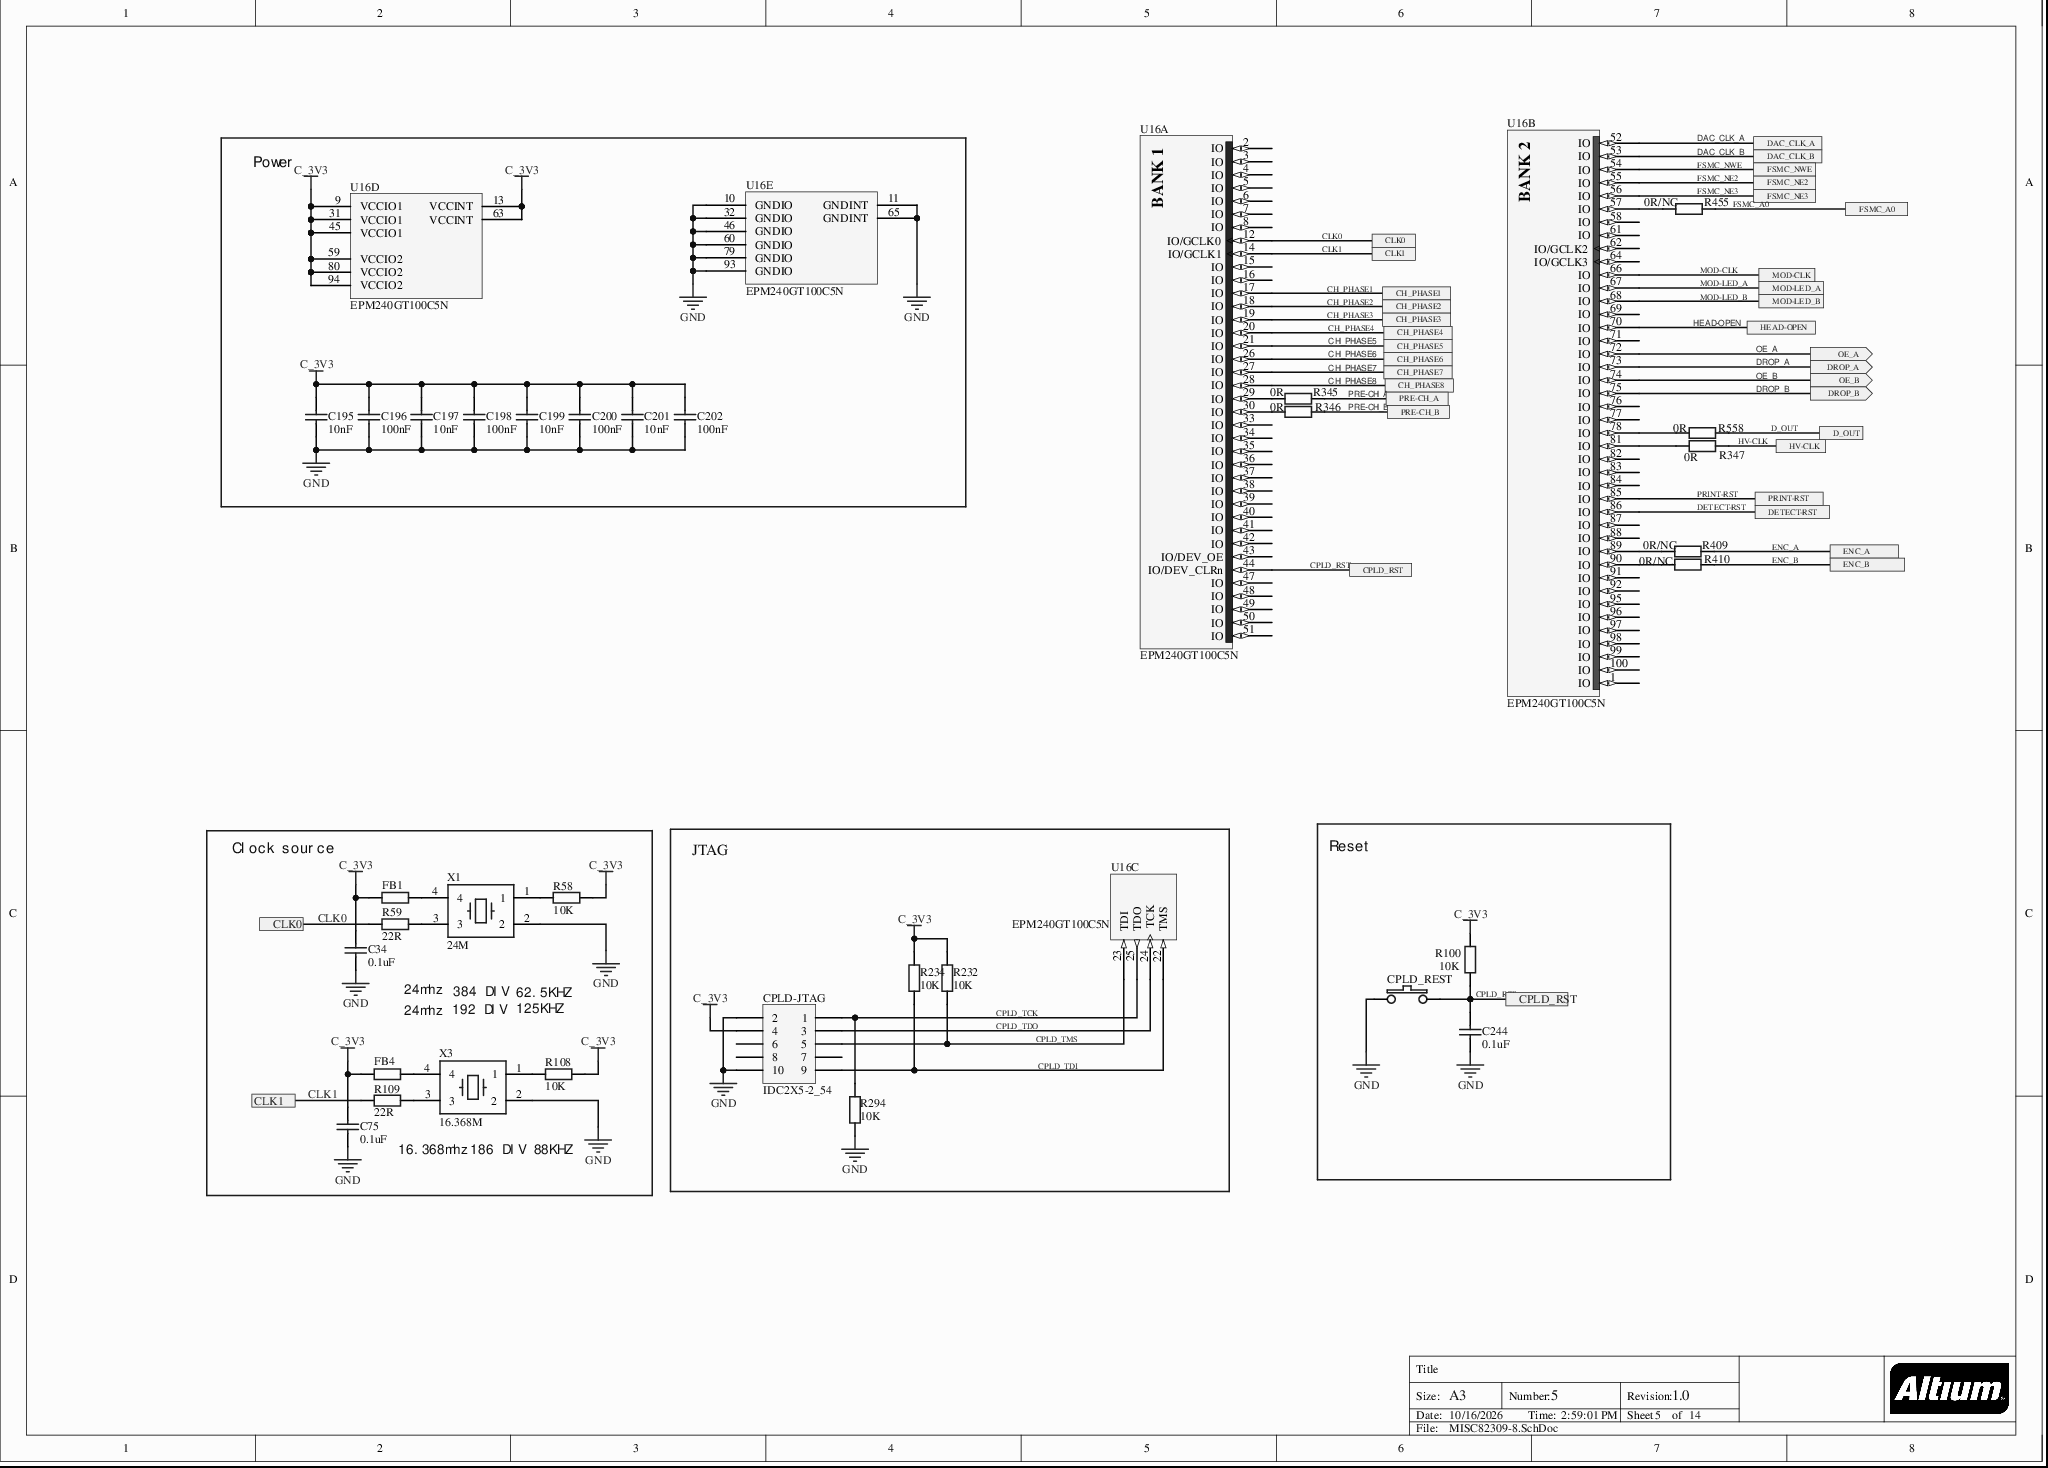
[diagram p0: MISC82309-8.SchDoc]
# Altium project MISC82309-16.PrjPcb (part 3 of 6)

## Sheet MISC82309-8.SchDoc
size A3; DocumentNumber: 5; Revision: 1.0; SheetNumber: 5; SheetTotal: 14

### Parts
C34  0.1uF  [C0603]
C75  0.1uF  [C0603]
C195  10nF  [C0805]
C196  100nF  [C0805]
C197  10nF  [C0805]
C198  100nF  [C0805]
C199  10nF  [C0805]
C200  100nF  [C0805]
C201  10nF  [C0805]
C202  100nF  [C0805]
C244  0.1uF  [C0603]
CPLD-JTAG  IDC2X5-2_54  [IDC2X5-2_54]
CPLD_REST  SW  [SW-6X3X2.5]  (value not drawn)
FB1  60  [SMD1206-L]  (value not drawn)
FB4  60  [SMD1206-L]  (value not drawn)
R58  10K  [R0603]
R59  22R  [R0603]
R100  10K  [R0603]
R108  10K  [R0603]
R109  22R  [R0603]
R232  10K  [R0603]
R234  10K  [R0603]
R294  10K  [R0603]
R345  0R  [RES_0603]
R346  0R  [RES_0603]
R347  0R  [RES_0603]
R409  0R/NC  [RES_0603]
R410  0R/NC  [RES_0603]
R455  0R/NC  [RES_0603]
R558  0R  [RES_0603]
U16  EPM240GT100C5N  [TQFP100_N]  (parts A,B,C,D,E of 5)
X1  24M  [SMD5032]
X3  16.368M  [SMD5032]

### Blocks framed on the sheet
Power: C195-C202 U16
Clock source: C34 C75 FB1 FB4 R58 R59 R108 R109 X1 X3
JTAG: CPLD-JTAG R232 R234 R294 U16
Reset: C244 CPLD_REST R100

### Ports
CH_PHASE1, CH_PHASE2, CH_PHASE3, CH_PHASE4, CH_PHASE5, CH_PHASE6, CH_PHASE7, CH_PHASE8, CLK0, CLK1, CPLD_RST, D_OUT, DAC_CLK_A, DAC_CLK_B, DETECT-RST, DROP_A (out), DROP_B (out), ENC_A, ENC_B, FSMC_A0, FSMC_NE2, FSMC_NE3, FSMC_NWE, HEAD-OPEN, HV-CLK, MOD-CLK, MOD-LED_A, MOD-LED_B, OE_A (out), OE_B (out), PRE-CH_A, PRE-CH_B, PRINT-RST

### Nets
C_3V3: C34.2 C75.2 C195.2 C196.2 C197.2 C198.2 C199.2 C200.2 C201.2 C202.2 CPLD-JTAG.4 FB1.1 FB4.1 R58.2 R100.1 R108.2 R232.2 R234.2 U16.9(VCCIO1) U16.13(VCCINT) U16.31(VCCIO1) U16.45(VCCIO1) U16.59(VCCIO2) U16.63(VCCINT) U16.80(VCCIO2) U16.94(VCCIO2)
GND: C34.1 C75.1 C195.1 C196.1 C197.1 C198.1 C199.1 C200.1 C201.1 C202.1 C244.1 CPLD-JTAG.2 CPLD-JTAG.10 CPLD_REST.1 R294.1 U16.10(GNDIO) U16.11(GNDINT) U16.32(GNDIO) U16.46(GNDIO) U16.60(GNDIO) U16.65(GNDINT) U16.79(GNDIO) U16.93(GNDIO) X1.2 X3.2
CH_PHASE1: U16.17(IO) ; port CH_PHASE1
CH_PHASE2: U16.18(IO) ; port CH_PHASE2
CH_PHASE3: U16.19(IO) ; port CH_PHASE3
CH_PHASE4: U16.20(IO) ; port CH_PHASE4
CH_PHASE5: U16.21(IO) ; port CH_PHASE5
CH_PHASE6: U16.26(IO) ; port CH_PHASE6
CH_PHASE7: U16.27(IO) ; port CH_PHASE7
CH_PHASE8: U16.28(IO) ; port CH_PHASE8
CLK0: R59.1 U16.12(IO/GCLK0) ; port CLK0
CLK1: R109.1 U16.14(IO/GCLK1) ; port CLK1
CPLD_RST: C244.2 CPLD_REST.2 R100.2 U16.44(IO/DEV_CLRn) ; port CPLD_RST
CPLD_TCK: CPLD-JTAG.1 R294.2 U16.25(TDO)
CPLD_TDI: CPLD-JTAG.9 R234.1 U16.22(TMS)
CPLD_TDO: CPLD-JTAG.3 U16.24(TCK)
CPLD_TMS: CPLD-JTAG.5 R232.1 U16.23(TDI)
D_OUT: R558.1 ; port D_OUT
DAC_CLK_A: U16.52(IO) ; port DAC_CLK_A
DAC_CLK_B: U16.53(IO) ; port DAC_CLK_B
DETECT-RST: U16.86(IO) ; port DETECT-RST
DROP_A: U16.73(IO) ; port DROP_A
DROP_B: U16.75(IO) ; port DROP_B
ENC_A: R409.2 ; port ENC_A
ENC_B: R410.2 ; port ENC_B
FSMC_A0: R455.2 ; port FSMC_A0
FSMC_NE2: U16.55(IO) ; port FSMC_NE2
FSMC_NE3: U16.56(IO) ; port FSMC_NE3
FSMC_NWE: U16.54(IO) ; port FSMC_NWE
HEAD-OPEN: U16.70(IO) ; port HEAD-OPEN
HV-CLK: R347.2 ; port HV-CLK
MOD-CLK: U16.66(IO) ; port MOD-CLK
MOD-LED_A: U16.67(IO) ; port MOD-LED_A
MOD-LED_B: U16.68(IO) ; port MOD-LED_B
OE_A: U16.72(IO) ; port OE_A
OE_B: U16.74(IO) ; port OE_B
PRE-CH_A: R345.2 ; port PRE-CH_A
PRE-CH_B: R346.2 ; port PRE-CH_B
PRINT-RST: U16.85(IO) ; port PRINT-RST
NetFB1_2: FB1.2 X1.4
NetFB4_2: FB4.2 X3.4
NetR58_1: R58.1 X1.1
NetR59_2: R59.2 X1.3
NetR108_1: R108.1 X3.1
NetR109_2: R109.2 X3.3
NetR345_1: R345.1 U16.29(IO)
NetR346_1: R346.1 U16.30(IO)
NetR347_1: R347.1 U16.81(IO)
NetR409_1: R409.1 U16.89(IO)
NetR410_1: R410.1 U16.90(IO)
NetR455_1: R455.1 U16.57(IO)
NetR558_2: R558.2 U16.78(IO)

Not connected (* = marked no-connect by the designer): CPLD-JTAG 6 7 8; CPLD_REST 5 6; U16 1(IO) 2(IO) 3(IO) 4(IO) 5(IO) 6(IO) 7(IO) 8(IO) 15(IO) 16(IO) 33(IO) 34(IO) 35(IO) 36(IO) 37(IO) 38(IO) 39(IO) 40(IO) 41(IO) 42(IO) 43(IO/DEV_OE) 47(IO) 48(IO) 49(IO) 50(IO) 51(IO) 58(IO) 61(IO) 62(IO/GCLK2) 64(IO/GCLK3) 69(IO) 71(IO) 76(IO) 77(IO) 82(IO) 83(IO) 84(IO) 87(IO) 88(IO) 91(IO) 92(IO) 95(IO) 96(IO) 97(IO) 98(IO) 99(IO) 100(IO)

### Notes on the sheet
- 24mhz
- 192 DIV
- 384 DIV
- 125KHZ
- 62.5KHZ
- 16.368mhz
- (near X3) 186 DIV
- 88KHZ
- Title
- Size:
- Date:
- A3
- Number:
- Time:
- Revision:
- Sheet
- of
- File:

### Library data of the parts
C34 C75 C195 C197 C199 C201 C244 = CAP_1206: Capacitor
  C34 C75 C244: value: 0.1uF
  C195 C197 C199 C201: value: 10nF
C196 C198 C200 C202 = CAP_1206: Capacitor; value: 0.1uF
CPLD-JTAG = HEAD2X5-2_54
FB1 FB4 = FB: Res; value: 10K
R58 R108 R232 R234 R294 = Res: value: 10K
R59 R109 = Res: value: 22ohm
R100 = Res2: Resistor; Published: 8-Jun-2000; LatestRevisionDate: 17-Jul-2002; LatestRevisionNote: Re-released for DXP Platform.; PackageReference: AXIAL-0.4; Value: 10K; Publisher: Altium Limited
R345-R347 = Res_0603: Res; value: 0R
R409 R410 R455 = Res_0603: Res; value: 0R
R558 = Res_0603: Res; value: 0R/NC
U16 = EPM240GT100C5N: MAX II 1.8V CPLD, 80 IOs, 240 Logic Elements, 100-Pin Plastic TQFP, Commercial Temperature, Speed Grade 5, Pb-Free; Note: Each set of VCCIO pins can be connected to 3.3V, 2.5V, 1.8V, or 1.5V.; Note: All VCCINT pins must be connected to 1.8V.; Published: 4-Mar-2005; LatestRevisionDate: 13-Apr-2006; LatestRevisionNote: IPC-7351 Footprint Added.; DatasheetVersion: ver1.8, Jul-2006; PackageVersion: ver14.3, Jul-2006; PackageReference: TQFP100; PackageDescription: 100-Pin Plastic Thin Quad Flat Pack (TQFP100); Code_JEDEC: MS-026-AED; ComponentLink1Description: Manufacturer Link; ComponentLink1URL: http://www.altera.com/products/devices/cpld/max2/mx2-index.jsp; ComponentLink2Description: Handbook; ComponentLink2URL: http://www.altera.com/literature/hb/max2/max2_mii5v1.pdf; ComponentLink3Description: Packaging Specification; ComponentLink3URL: http://www.altera.com/literature/ds/dspkg.pdf; Publisher: Altium Limited
X1 X3 = SOC_24M

## Sheet MISC82309-13.SchDoc
size A3; DocumentNumber: 6; Revision: 1.0; SheetNumber: 6; SheetTotal: 14
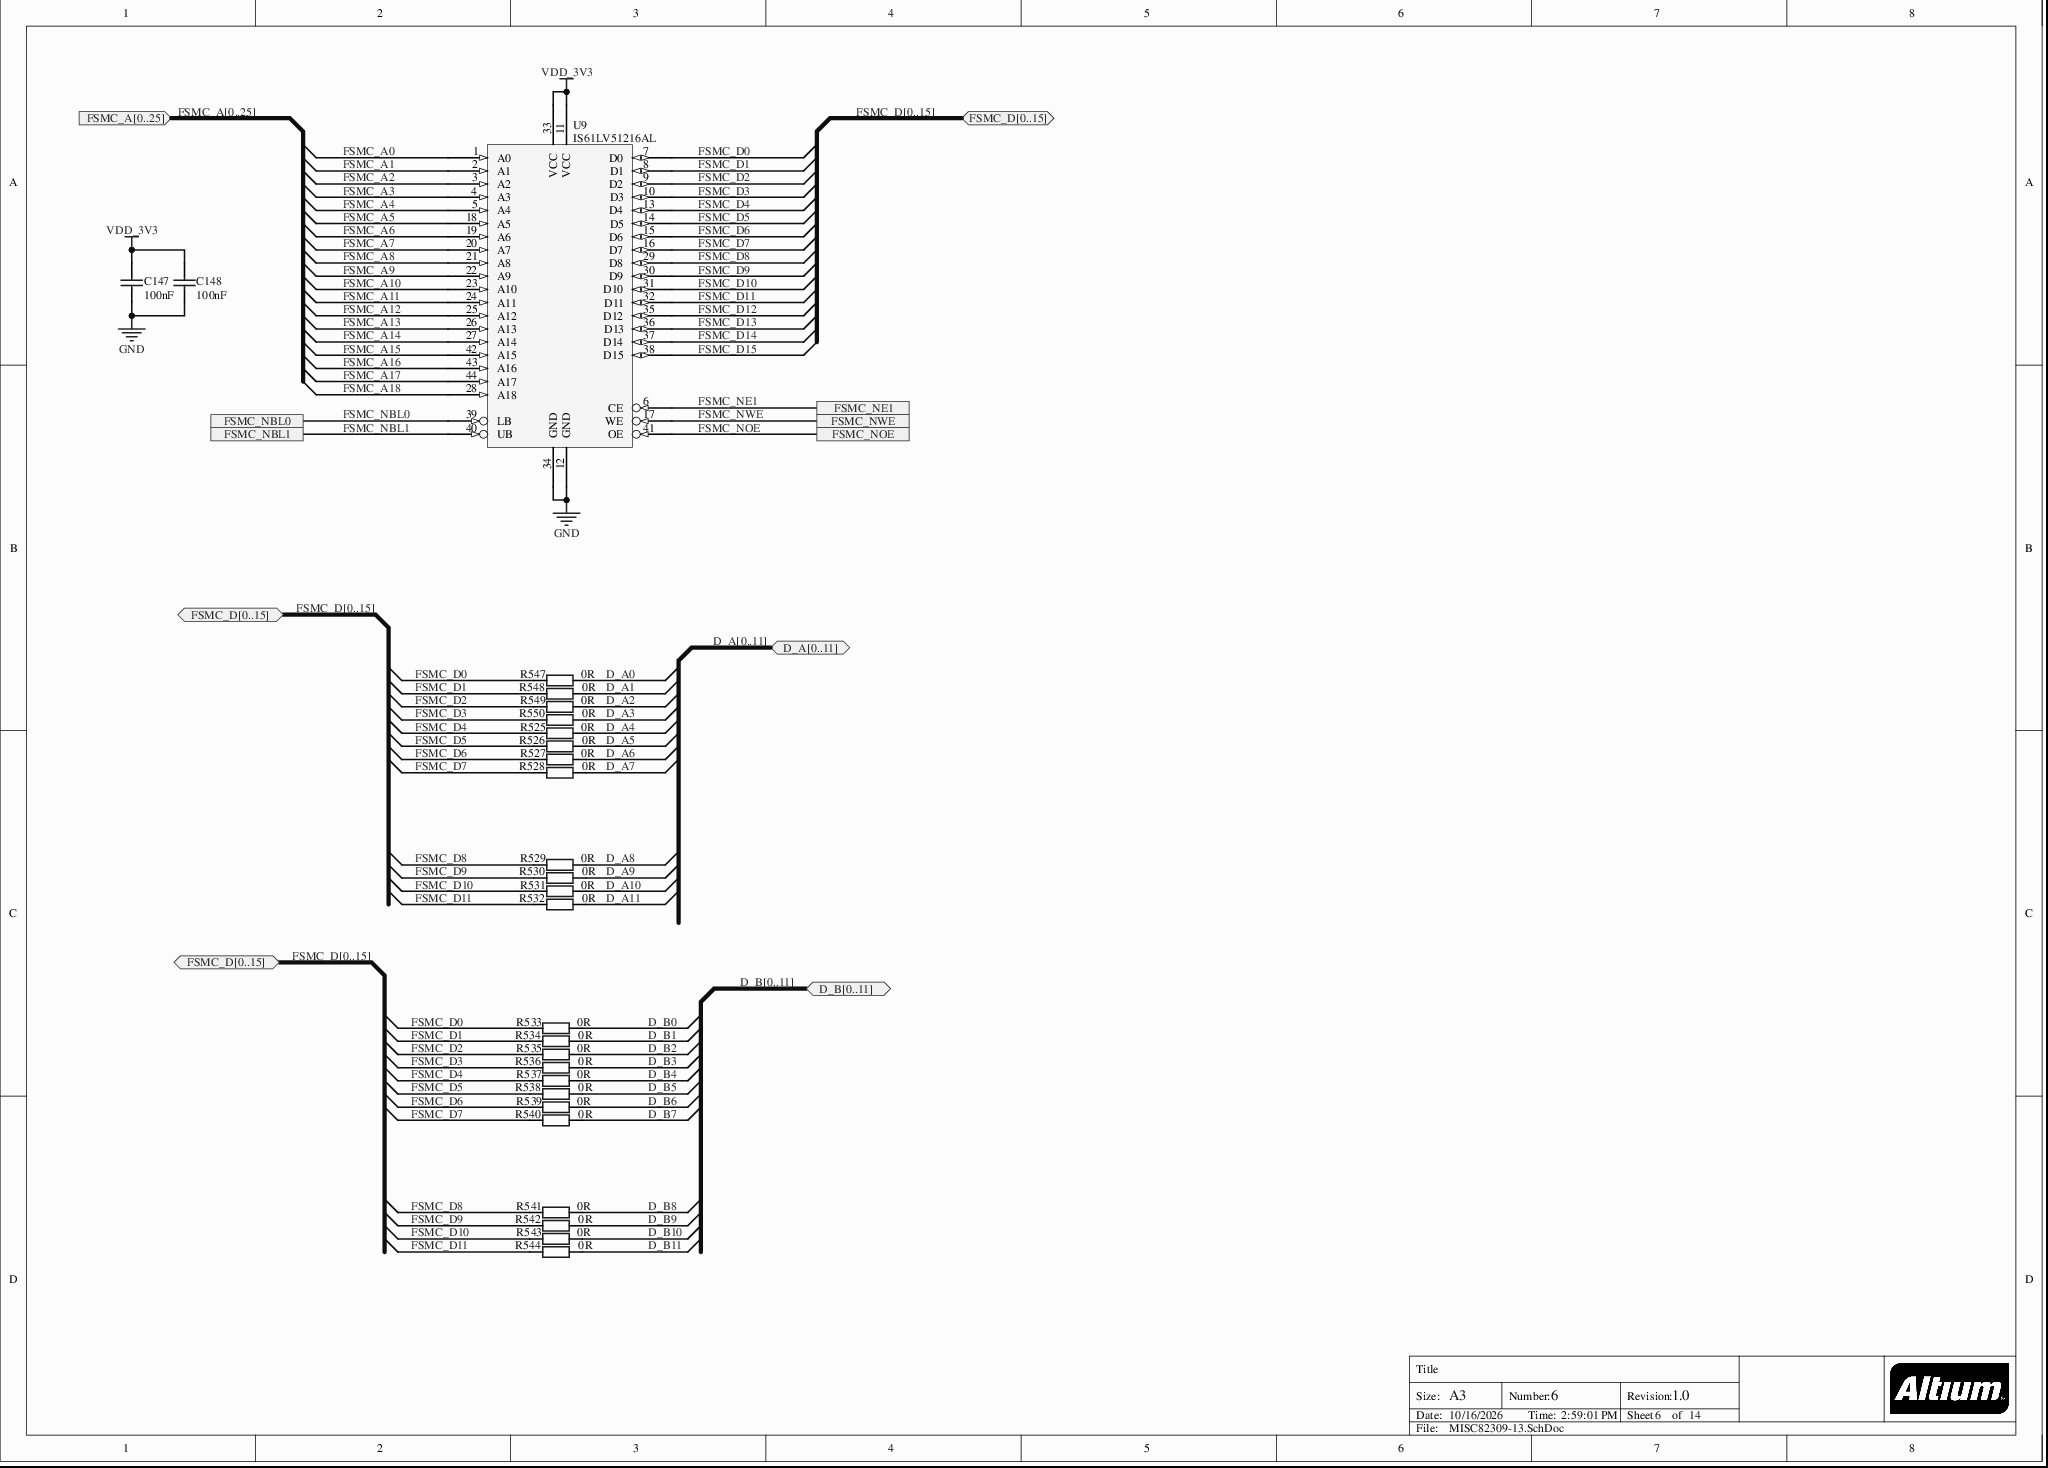
[diagram p1: MISC82309-13.SchDoc]

### Parts
C147  100nF  [C0603]
C148  100nF  [C0603]
R525  0R  [RES_0603]
R526  0R  [RES_0603]
R527  0R  [RES_0603]
R528  0R  [RES_0603]
R529  0R  [RES_0603]
R530  0R  [RES_0603]
R531  0R  [RES_0603]
R532  0R  [RES_0603]
R533  0R  [RES_0603]
R534  0R  [RES_0603]
R535  0R  [RES_0603]
R536  0R  [RES_0603]
R537  0R  [RES_0603]
R538  0R  [RES_0603]
R539  0R  [RES_0603]
R540  0R  [RES_0603]
R541  0R  [RES_0603]
R542  0R  [RES_0603]
R543  0R  [RES_0603]
R544  0R  [RES_0603]
R547  0R  [RES_0603]
R548  0R  [RES_0603]
R549  0R  [RES_0603]
R550  0R  [RES_0603]
U9  IS61LV51216AL  [TSOP44-IS61LV51216AL-10TLI]

### Ports
D_A[0..11] (bidir), D_B[0..11] (bidir), FSMC_A[0..25] (in), FSMC_D[0..15] (bidir), FSMC_NBL0, FSMC_NBL1, FSMC_NE1, FSMC_NOE, FSMC_NWE

### Nets
GND: C147.1 C148.1 U9.12(GND) U9.34(GND)
VDD_3V3: C147.2 C148.2 U9.11(VCC) U9.33(VCC)
D_A0: R547.1
D_A1: R548.1
D_A2: R549.1
D_A3: R550.1
D_A4: R525.1
D_A5: R526.1
D_A6: R527.1
D_A7: R528.1
D_A8: R529.1
D_A9: R530.1
D_A10: R531.1
D_A11: R532.1
D_B0: R533.1
D_B1: R534.1
D_B2: R535.1
D_B3: R536.1
D_B4: R537.1
D_B5: R538.1
D_B6: R539.1
D_B7: R540.1
D_B8: R541.1
D_B9: R542.1
D_B10: R543.1
D_B11: R544.1
FSMC_A0: U9.1(A0)
FSMC_A1: U9.2(A1)
FSMC_A2: U9.3(A2)
FSMC_A3: U9.4(A3)
FSMC_A4: U9.5(A4)
FSMC_A5: U9.18(A5)
FSMC_A6: U9.19(A6)
FSMC_A7: U9.20(A7)
FSMC_A8: U9.21(A8)
FSMC_A9: U9.22(A9)
FSMC_A10: U9.23(A10)
FSMC_A11: U9.24(A11)
FSMC_A12: U9.25(A12)
FSMC_A13: U9.26(A13)
FSMC_A14: U9.27(A14)
FSMC_A15: U9.42(A15)
FSMC_A16: U9.43(A16)
FSMC_A17: U9.44(A17)
FSMC_A18: U9.28(A18)
FSMC_D0: R533.2 R547.2 U9.7(D0)
FSMC_D1: R534.2 R548.2 U9.8(D1)
FSMC_D2: R535.2 R549.2 U9.9(D2)
FSMC_D3: R536.2 R550.2 U9.10(D3)
FSMC_D4: R525.2 R537.2 U9.13(D4)
FSMC_D5: R526.2 R538.2 U9.14(D5)
FSMC_D6: R527.2 R539.2 U9.15(D6)
FSMC_D7: R528.2 R540.2 U9.16(D7)
FSMC_D8: R529.2 R541.2 U9.29(D8)
FSMC_D9: R530.2 R542.2 U9.30(D9)
FSMC_D10: R531.2 R543.2 U9.31(D10)
FSMC_D11: R532.2 R544.2 U9.32(D11)
FSMC_D12: U9.35(D12)
FSMC_D13: U9.36(D13)
FSMC_D14: U9.37(D14)
FSMC_D15: U9.38(D15)
FSMC_NBL0: U9.39(LB) ; port FSMC_NBL0
FSMC_NBL1: U9.40(UB) ; port FSMC_NBL1
FSMC_NE1: U9.6(CE) ; port FSMC_NE1
FSMC_NOE: U9.41(OE) ; port FSMC_NOE
FSMC_NWE: U9.17(WE) ; port FSMC_NWE

### Buses and harness runs
bus D_A[0..11] = port D_A[0..11]
bus D_B[0..11] = port D_B[0..11]
bus FSMC_A[0..25] = port FSMC_A[0..25]
bus FSMC_D[0..15] = port FSMC_D[0..15]

### Notes on the sheet
- Title
- Size:
- Date:
- A3
- Number:
- Time:
- Revision:
- Sheet
- of
- File:

### Library data of the parts
C147 C148 = CAP_1206: Capacitor; value: 0.1uF
R525-R544 R547-R550 = Res_0603: Res; value: 0R/NC

## Sheet MISC82309-12.SchDoc
size A3; DocumentNumber: 7; Revision: 1.0; SheetNumber: 7; SheetTotal: 14
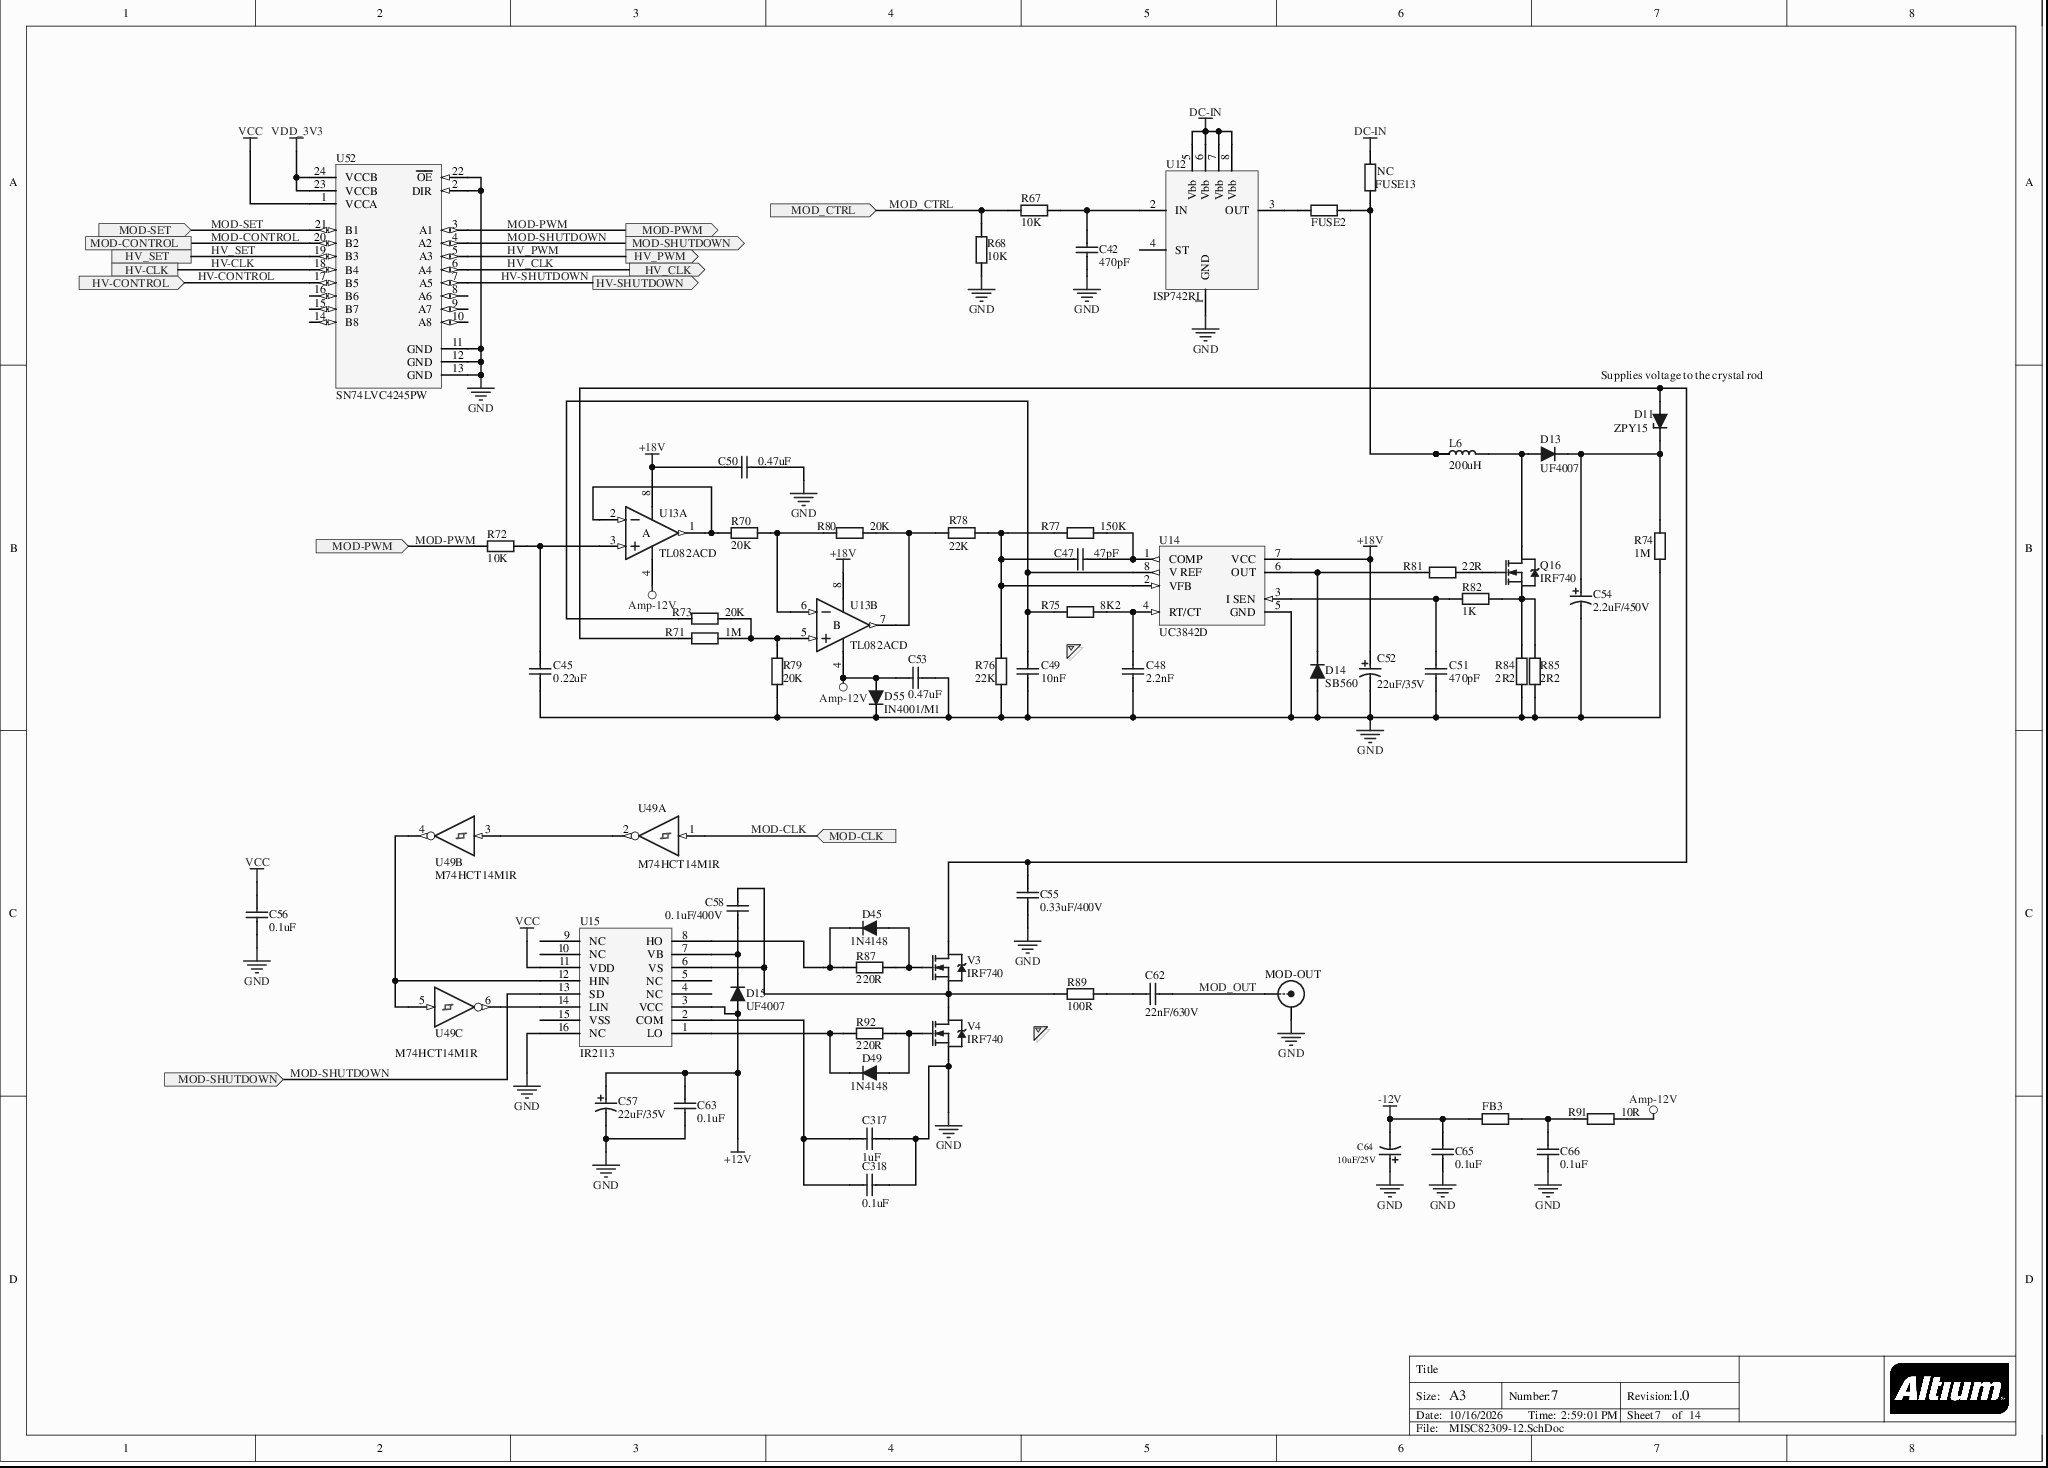
[diagram p2: MISC82309-12.SchDoc]

### Parts
C42  470pF  [C0603]
C45  0.22uF  [C1206]
C47  47pF  [C1206]
C48  2.2nF  [C1206]
C49  10nF  [C1206]
C50  0.47uF  [C1206]
C51  470pF  [C1206]
C52  22uF/35V  [E6.3X5.4]
C53  0.47uF  [C1206]
C54  2.2uF/450V  [CAP-EL-10X13_5-5]
C55  0.33uF/400V  [CBB-400V-10mm]
C56  0.1uF  [CAP_0805]
C57  22uF/35V  [CAP_AVX-A]
C58  0.1uF/400V  [CBB-400V-10mm]
C62  22nF/630V  [CBB-400V-10mm]
C63  0.1uF  [C1206]
C64  10uF/25V  [E5X5.4]
C65  0.1uF  [C0805]
C66  0.1uF  [C0805]
C317  1uF  [CAP_0805]
C318  0.1uF  [CAP_0805]
D11  ZPY15  [DO-41 - 10.46mm]
D13  UF4007  [DO-41 - 10.46mm]
D14  SB560  [DO-201AD]
D15  UF4007  [DO-41 - 10.46mm]
D45  1N4148  [DO-213AA]
D49  1N4148  [DO-213AA]
D55  IN4001/M1  [DO-214AC]
FB3  60  [SMD0805-L]  (value not drawn)
FUSE2  ASMD050-1812(30V,0.5A)  [SMD1812-Fuse]  (value not drawn)
FUSE13  value NC  [SMD1812-Fuse]  (hidden comment: ASMD050-1812(30V,0.5A))
L6  200uH  [L200/1.4A]
MOD-OUT  SMB  [SMB_V-RJ45]  (value not drawn)
Q16  IRF740  [TO220V1]
R67  10K  [R0603]
R68  10K  [R0603]
R70  20K  [R1206]
R71  1M  [R1206]
R72  10K  [R1206]
R73  20K  [R1206]
R74  1M  [R1206]
R75  8K2  [R1206]
R76  22K  [R1206]
R77  150K  [R1206]
R78  22K  [R1206]
R79  20K  [R1206]
R80  20K  [R1206]
R81  22R  [R1206]
R82  1K  [R1206]
R84  2R2  [R1206]
R85  2R2  [R1206]
R87  220R  [R1206]
R89  100R  [RES_2512]
R91  10R  [RES_0805]
R92  220R  [R1206]
U12  ISP742RI  [P-DSO-8]
U13  TL082ACD  [SO8]  (parts A,B of 2)
U14  UC3842D  [SOIC-8]
U15  IR2113  [SOIC-16]
U49  M74HCT14M1R  [SO14]  (parts A,B,C of 6)
U52  SN74LVC4245PW  [TSSOP-24]
V3  IRF740  [TO220V1]
V4  IRF740  [TO220V1]

### Ports
HV-CLK, HV-CONTROL (in), HV-SHUTDOWN (out), HV_CLK (out), HV_PWM (out), HV_SET, MOD-CLK (in), MOD-CONTROL, MOD-PWM (in), MOD-PWM (out), MOD-SET (in), MOD-SHUTDOWN (in), MOD-SHUTDOWN (out), MOD_CTRL (in)

### Nets
+12V: C57.1 C63.2 D15.1 U15.3(VCC)
+18V: C50.1 C52.1 U13.8(V+) U14.7(VCC)
-12V: C64.2 C65.2 FB3.1
Amp-12V: C53.1 D55.1 R91.2 U13.4(V-)
DC-IN: FUSE13.1 U12.5(Vbb) U12.6(Vbb) U12.7(Vbb) U12.8(Vbb)
GND: C42.1 C45.2 C48.2 C49.2 C50.2 C51.2 C52.2 C53.2 C54.2 C55.1 C56.2 C57.2 C63.1 C64.1 C65.1 C66.1 C317.2 C318.2 D14.1 D55.2 MOD-OUT.2(Y) R68.1 R74.1 R76.1 R79.1 R84.1 R85.1 U12.1(GND) U14.5(GND) U15.16(NC) U49.7(GND) U52.2(DIR) U52.11(GND) U52.12(GND) U52.13(GND) U52.22(~{OE}) V4.3(S)
VCC: C56.1 U15.11(VDD) U49.14(VCC) U52.1(VCCA)
VDD_3V3: U52.23(VCCB) U52.24(VCCB)
HV-CLK: U52.18(B4) ; port HV-CLK
HV-CONTROL: U52.17(B5) ; port HV-CONTROL
HV-SHUTDOWN: U52.7(A5) ; port HV-SHUTDOWN
HV_CLK: U52.6(A4) ; port HV_CLK
HV_PWM: U52.5(A3) ; port HV_PWM
HV_SET: U52.19(B3) ; port HV_SET
MOD-CLK: U49.1(A) ; port MOD-CLK
MOD-CONTROL: U52.20(B2) ; port MOD-CONTROL
MOD-PWM: R72.2 U52.3(A1) ; port MOD-PWM
MOD-SET: U52.21(B1) ; port MOD-SET
MOD-SHUTDOWN: U15.13(SD) U52.4(A2) ; port MOD-SHUTDOWN
MOD_CTRL: R67.2 R68.2 ; port MOD_CTRL
MOD_OUT: C62.2 MOD-OUT.1(X)
NetC42_2: C42.2 R67.1 U12.2(IN)
NetC45_1: C45.1 R72.1 U13.3(IN+)
NetC47_1: C47.1 R77.2 U14.1(COMP)
NetC47_2: C47.2 R76.2 R77.1 R78.2 U14.2(VFB)
NetC48_1: C48.1 R75.2 U14.4(RT/CT)
NetC49_1: C49.1 R73.1 R75.1 U14.8(V_REF)
NetC51_1: C51.1 R82.1 U14.3(I_SEN)
NetC54_1: C54.1 D11.2 D13.2 R74.2
NetC55_2: C55.2 D11.1 R71.1 V3.2(D)
NetC58_1: C58.1 R89.1 U15.6(VS) V3.3(S) V4.2(D)
NetC58_2: C58.2 D15.2 U15.7(VB)
NetC62_1: C62.1 R89.2
NetC66_2: C66.2 FB3.2 R91.1
NetC317_1: C317.1 C318.1 U15.2(COM)
NetD13_1: D13.1 L6.2 Q16.2(D)
NetD14_2: D14.2 R81.1 U14.6(OUT)
NetD45_1: D45.1 R87.1 V3.1(G)
NetD45_2: D45.2 R87.2 U15.8(HO)
NetD49_1: D49.1 R92.1 V4.1(G)
NetD49_2: D49.2 R92.2 U15.1(LO)
NetFUSE2_1: FUSE2.1 U12.3(OUT)
NetFUSE2_2: FUSE2.2 FUSE13.2 L6.1 L6.3
NetQ16_1: Q16.1(G) R81.2
NetQ16_3: Q16.3(S) R82.2 R84.2 R85.2
NetR70_1: R70.1 U13.1(OUT) U13.2(IN-)
NetR70_2: R70.2 R80.1 U13.6(IN-)
NetR71_2: R71.2 R73.2 R79.2 U13.5(IN+)
NetR78_1: R78.1 R80.2 U13.7(OUT)
NetU15_12: U15.12(HIN) U49.4(Y) U49.5(A)
NetU15_14: U15.14(LIN) U49.6(Y)
NetU49_2: U49.2(Y) U49.3(A)

Not connected (* = marked no-connect by the designer): U12 4(ST); U15 4(NC) 5(NC) 9(NC) 10(NC) 15(VSS); U52 8(A6) 9(A7) 10(A8) 14(B8) 15(B7) 16(B6)

### Notes on the sheet
- (near D11) Supplies voltage to the crystal rod
- C8=2.2nF，代表死区时间是0.7us左右，RT》5K
  振荡器频率fo(khz)=1.72/(RT(K)*CT(uF))=95.3Khz
  RT=R13,CT=C8
- HO:幅值35V的62.5KHZ的方波
  LO:幅值12V的62.5KHZ的方波
  V3与V4连接处：幅值25V的62.5KHZ的方波：
  晶振电压MOD_OUT:+-12V的62.5KHZ方波
- Title
- Size:
- Date:
- A3
- Number:
- Time:
- Revision:
- Sheet
- of
- File:

### Library data of the parts
C42 = CAP_0.1uF: value: 470pF
C45 = CAP_0.22uF: Capacitor 0.22uF; AEMS Code: 2100341; value: 0.22uF
C47 = CAP_47pF: Capacitor 47pF; Value: 47pF
C48 = CAP_2.2nF: Capacitor 2.2nF; Value: 2.2nF
C49 = CAP_10nF: Capacitor 10nF; Value: 10nF
C50 C53 = CAP_0.47uF: Capacitor 0.47uF; AEMS Code: 2100341; value: 0.47uF
C51 = CAP_470pF: Capacitor 470pF; Value: 470pF
C52 = CAP_POLAR_22uF_35V: Polar Capacitor 22uF 35V; Value: 22uF/35V
C54 = CAP_POLAR_2.2uF_450V: Polar Capacitor 222uF 450V; Value: 2.2uF/450V
C55 = CAP_CBB_0.33uF_400V: CBB Capacitor 0.33uF 400V; Value: 0.33uF/400V
C56 C63 C317 C318 = CAP_0.1uF: Capacitor 0.1uF
  C56 C63 C318: Value: 0.1uF
  C317: Value: 1uF
C57 = CAP_AVX_4.7uF_16V: AVX Capacitor 4.7uFF 16V; Value: 22uF/35V
C58 = CAP_CBB_0.1uF_400V: CBB Capacitor0.1uF 400V; Value: 0.1uF/400V
C62 = CAP_CBB_22nF_630V: CBB Capacitor 22nF 630V; Value: 22nF/630V
C64 = CAP_POLAR_1: Polar Capacitor
C65 C66 = CAP_1206: Capacitor; value: 0.1uF
D55 = 1N4001/M1
FB3 = FB: Res; value: 10K
FUSE2 = FUSE: Res; Value: 30V/500mA
FUSE13 = FUSE: Res
L6 = Toroidal Inductor
MOD-OUT = SMB: SMB Straight Connector; LatestRevisionDate: 17-Jul-2002; LatestRevisionNote: Re-released for DXP Platform.; Publisher: Altium Limited
Q16 V3 V4 = IRF740: HEXFET N-Channel Power MOSFET; Note: Pin 2 is electrically connected to pin 4.; Published: 8-Jun-2000; LatestRevisionDate: 17-Jul-2002; LatestRevisionNote: Re-released for DXP Platform.; DatasheetVersion: PD-9.375H; PackageVersion: Feb-1997; PackageReference: TO-220AB; PackageDescription: TO, Thru-Hole, Vertical, Heatsink Mounted; 3 In-Line Leads; Pitch 2.54 mm; ComponentLink1Description: Manufacturer Link; ComponentLink1URL: http://www.irf.com/; ComponentLink2Description: Datasheet; ComponentLink2URL: http://www.irf.com/product-info/datasheets/data/irf740.pdf; Publisher: Altium Limited
R67 R68 R72 R91 = Res2: Resistor; Published: 8-Jun-2000; LatestRevisionDate: 17-Jul-2002; LatestRevisionNote: Re-released for DXP Platform.; PackageReference: AXIAL-0.4; Publisher: Altium Limited
  R67 R68 R72: Value: 10K
  R91: Value: 10R
R70 R73 R79 R80 = Res_20K: value: 20K
R71 R74 = Res_1M: Resistance 1M; value: 1M
R75 = Res_8K2: value: 8K2
R76 R78 = Res_22K: value: 22K
R77 = Res_150K: value: 150K
R81 = Res_22R: value: 22R
R82 = Res_1K: Resistance 1K; value: 1K
R84 = Res_2R2: value: 2R2
R85 = Res_1R: value: 2R2
R87 R92 = Res_220R: Resistance 220R; value: 220R
R89 = Res_100R: Resistance 100R; value: 100R
U12 = I742RI
U13 = TL082ACD: General-Purpose J-FET Dual Operational Amplifier; Published: 24-Aug-2001; LatestRevisionDate: 13-Apr-2006; LatestRevisionNote: IPC-7351 Footprint Added.; DatasheetVersion: Jan-1999; PackageVersion: Dec-2002; PackageReference: SO8; PackageDescription: 8-Pin Small Outline Integrated Circuit 1.27 mm Pitch; Code_JEDEC: MS-012-AA; Code_IPC: SOIC127P600-8; ComponentLink1Description: Manufacturer Link; ComponentLink1URL: http://www.st.com/; ComponentLink2Description: Datasheet; ComponentLink2URL: http://www.st.com/stonline/products/literature/ds/2300/tl082.pdf; Publisher: Altium Limited
U14 = UC3842N: Current Mode PWM Controller; PackageReference: SOIC-8
U15 = IR2110: High and Low Side Driver; PackageReference: SOIC-16
U49 = M74HCT14M1R: Hex Schmitt Inverter; Published: 8-Jun-2000; LatestRevisionDate: 13-Apr-2006; LatestRevisionNote: IPC-7351 Footprint Added.; DatasheetVersion: Oct-1993; PackageVersion: Sep-1998; PackageReference: SO14; PackageDescription: 14-Pin Small Outline Integrated Circuit 1.27 mm Pitch; Code_IPC: SOIC127P600-14; ComponentLink1Description: Manufacturer Link; ComponentLink1URL: http://www.st.com/; ComponentLink2Description: Datasheet; ComponentLink2URL: http://www.st.com/stonline/products/literature/ds/2106/m74hct14.pdf; Publisher: Altium Limited
U52 = SN74LVC4245PW: Octal Bus Transceiver and 3.3-V to 5-V Shifter with 3-State Outputs; Published: 8-Jun-2000; LatestRevisionDate: 04-Mar-2005; LatestRevisionNote: Stylized 3D Model Added.; DatasheetVersion: Jan-1997; PackageVersion: Feb-1999; PackageReference: PW024; PackageDescription: Shrink Small Outline; 24 Leads; Body Width 4.4 mm; Pitch 0.65 mm; ComponentLink1Description: Manufacturer Link; ComponentLink1URL: http://www.ti.com/; Publisher: Altium Limited
D11 = ZPY15: Supplier 1: Newark; Supplier Part Number 1: 22H4126
D14 = SB560: Supplier 1: Newark; Supplier Part Number 1: 05R5713